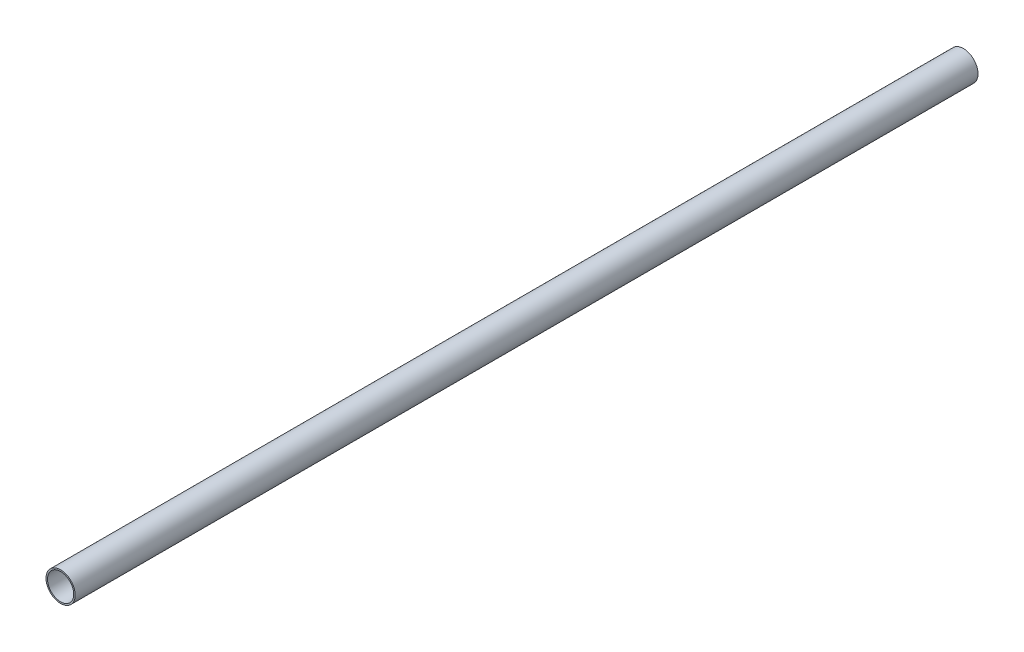
from build123d import *

# Parameters (mm, degrees)
SKETCH1_R           = 31.75
BOSS_EXTRUDE1_DEPTH = 1964
SHELL1_T            = -3.2


with BuildPart() as part:
    # Sketch1 → Boss-Extrude1 (new body)
    with BuildSketch(Plane.XY):
        with Locations(Location((0, 0, 0), (0, 0, 180))):
            Circle(SKETCH1_R)
    extrude(amount=BOSS_EXTRUDE1_DEPTH)

    # Shell1
    shell1_openings = [part.faces().sort_by_distance(p)[0] for p in [
        (0, 0, 1964),
        (0, 0, 0),
    ]]
    offset(amount=SHELL1_T, openings=shell1_openings, kind=Kind.INTERSECTION)


solid = part.part
